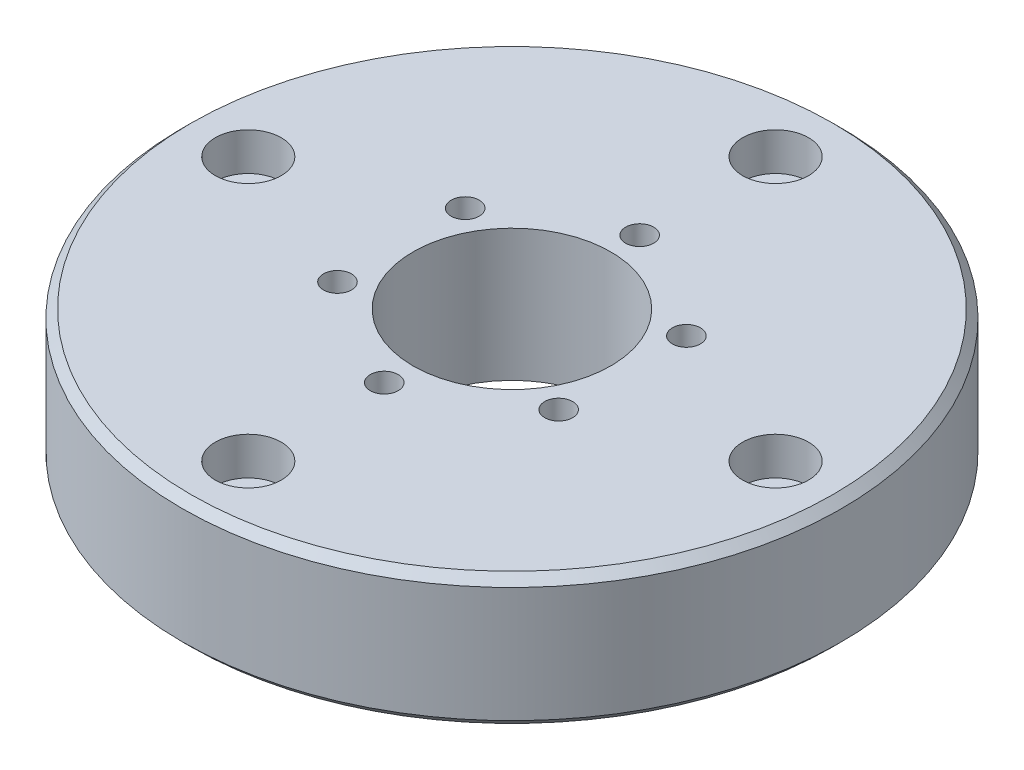
from build123d import *

# Parameters (mm, degrees)
SKETCH1_R                                          = 40
SKETCH1_R_2                                        = 12
BOSS_EXTRUDE1_DEPTH                                = 16
HOLE_SIZE_BASED_HEX_SOCKET_HEAD_CAP_SC_D           = 3.4
HOLE_SIZE_BASED_HEX_SOCKET_HEAD_CAP_SC_CBORE_D     = 6
HOLE_SIZE_BASED_HEX_SOCKET_HEAD_CAP_SC_CBORE_DEPTH = 3.4
HOLE_SIZE_BASED_HEX_SOCKET_HEAD_CA_2_D             = 4.5
HOLE_SIZE_BASED_HEX_SOCKET_HEAD_CA_2_CBORE_D       = 8
HOLE_SIZE_BASED_HEX_SOCKET_HEAD_CA_2_CBORE_DEPTH   = 4.6
CIRPATTERN1_COUNT                                  = 4
CHAMFER1_SIZE                                      = 1


with BuildPart() as part:
    # Sketch1 → Boss-Extrude1 (new body)
    with BuildSketch(Plane(origin=(0, 0, 0), x_dir=(1, 0, 0), z_dir=(0, 1, 0))):
        with Locations(Location((0, 0, 0), (0, 0, 270))):
            Circle(SKETCH1_R)
        with Locations(Location((0, 0, 0), (0, 0, 270))):
            Circle(SKETCH1_R_2, mode=Mode.SUBTRACT)
    extrude(amount=BOSS_EXTRUDE1_DEPTH)

    # Hole size _based_ hex socket head cap sc (through all)
    with Locations(Plane(origin=(0, 0, 0), x_dir=(-1, 0, 0), z_dir=(0, -1, 0))):
        with Locations((0, -15.5)):
            hole_size_based_hex_socket_head_cap_sc = CounterBoreHole(HOLE_SIZE_BASED_HEX_SOCKET_HEAD_CAP_SC_D / 2, HOLE_SIZE_BASED_HEX_SOCKET_HEAD_CAP_SC_CBORE_D / 2, HOLE_SIZE_BASED_HEX_SOCKET_HEAD_CAP_SC_CBORE_DEPTH)

    # SketchPattern1: Hole size _based_ hex socket head cap sc at 5 more places
    with Locations((13.423394, 0, -23.25), (13.423394, 0, -7.75), (-13.423394, 0, -7.75), (-13.423394, 0, -23.25), (0, 0, -31)):
        add(hole_size_based_hex_socket_head_cap_sc, mode=Mode.SUBTRACT)

    # Hole size _based_ hex socket head ca 2 (through all)
    with Locations(Plane(origin=(0, 16, 0), x_dir=(1, 0, 0), z_dir=(0, 1, 0))):
        with Locations((0, 32)):
            hole_size_based_hex_socket_head_ca_2 = CounterBoreHole(HOLE_SIZE_BASED_HEX_SOCKET_HEAD_CA_2_D / 2, HOLE_SIZE_BASED_HEX_SOCKET_HEAD_CA_2_CBORE_D / 2, HOLE_SIZE_BASED_HEX_SOCKET_HEAD_CA_2_CBORE_DEPTH)

    # CirPattern1: Hole size _based_ hex socket head ca 2 ×4 about axis
    cirpattern1_axis = Axis((0, 0, 0), (0, 1, 0))
    for i in range(1, CIRPATTERN1_COUNT):
        add(hole_size_based_hex_socket_head_ca_2.rotate(cirpattern1_axis, i * 360 / CIRPATTERN1_COUNT), mode=Mode.SUBTRACT)

    # Chamfer1
    chamfer1_edges = [part.edges().sort_by_distance(p)[0] for p in [
        (0, 0, -40),
        (0, 16, -40),
    ]]
    chamfer(chamfer1_edges, length=CHAMFER1_SIZE)


solid = part.part
